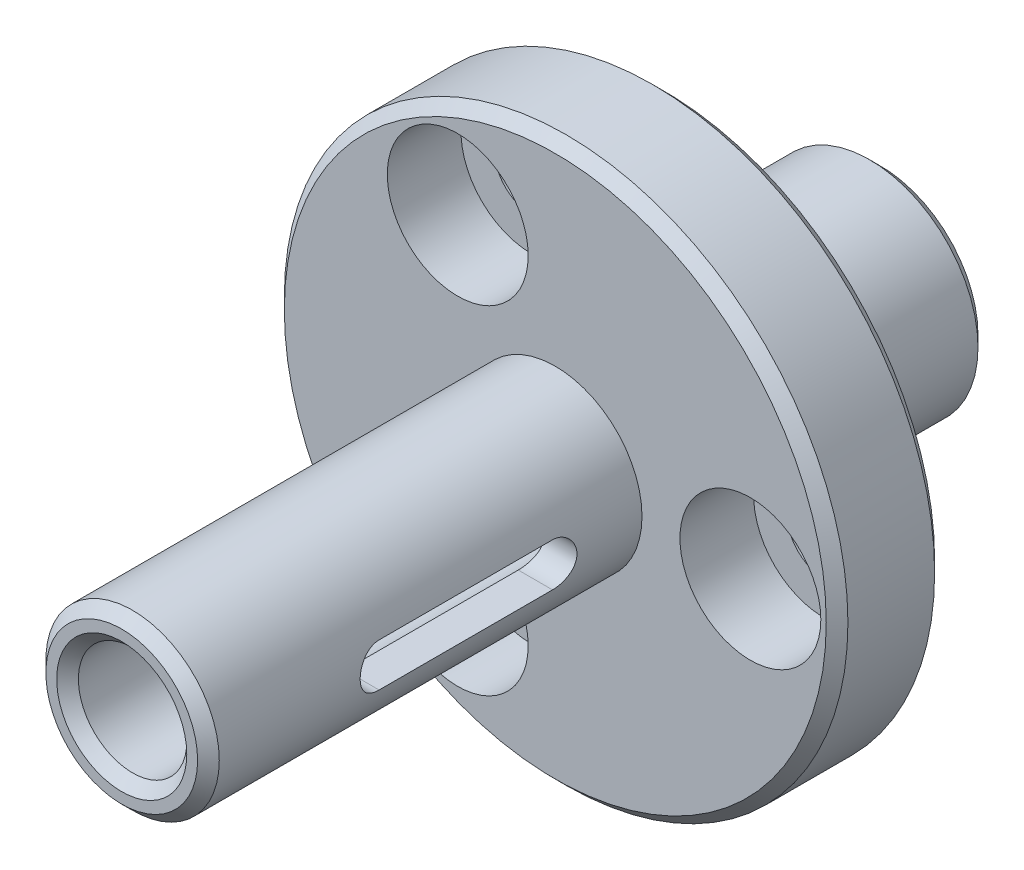
from build123d import *

# Parameters (mm, degrees)
SKETCH1_R                                           = 5
BOSS_EXTRUDE1_DEPTH                                 = 10
SKETCH2_R                                           = 13
BOSS_EXTRUDE2_DEPTH                                 = 5
SKETCH3_R                                           = 4
BOSS_EXTRUDE3_DEPTH                                 = 20
SKETCH4_R                                           = 2.5
CUT_EXTRUDE1_DEPTH                                  = 30
CBORE_FOR_M3_HEX_SOCKET_HEAD_CAP_SCREW1_D           = 3.4
CBORE_FOR_M3_HEX_SOCKET_HEAD_CAP_SCREW1_CBORE_D     = 6.5
CBORE_FOR_M3_HEX_SOCKET_HEAD_CAP_SCREW1_CBORE_DEPTH = 3.4
CIRPATTERN1_COUNT                                   = 3
CUT_EXTRUDE2_DEPTH                                  = 42.024382994
CHAMFER1_SIZE                                       = 0.5


with BuildPart() as part:
    # Sketch1 → Boss-Extrude1 (new body)
    with BuildSketch(Plane.XY):
        Circle(SKETCH1_R)
    extrude(amount=BOSS_EXTRUDE1_DEPTH)

    # Sketch2 → Boss-Extrude2 (add)
    with BuildSketch(Plane.XY.offset(10)):
        Circle(SKETCH2_R)
    extrude(amount=BOSS_EXTRUDE2_DEPTH)

    # Sketch3 → Boss-Extrude3 (add)
    with BuildSketch(Plane.XY.offset(15)):
        Circle(SKETCH3_R)
    extrude(amount=BOSS_EXTRUDE3_DEPTH)

    # Sketch4 → Cut-Extrude1 (cut)
    with BuildSketch(Plane.XY.offset(35)):
        Circle(SKETCH4_R)
    extrude(amount=-CUT_EXTRUDE1_DEPTH, mode=Mode.SUBTRACT)

    # CBORE for M3 Hex Socket Head Cap Screw1 (through all)
    with Locations(Plane.XY.offset(15)):
        with Locations((9, 0)):
            cbore_for_m3_hex_socket_head_cap_screw1 = CounterBoreHole(CBORE_FOR_M3_HEX_SOCKET_HEAD_CAP_SCREW1_D / 2, CBORE_FOR_M3_HEX_SOCKET_HEAD_CAP_SCREW1_CBORE_D / 2, CBORE_FOR_M3_HEX_SOCKET_HEAD_CAP_SCREW1_CBORE_DEPTH)

    # CirPattern1: CBORE for M3 Hex Socket Head Cap Screw1 ×3 about axis
    cirpattern1_axis = Axis((0, 0, 0), (0, 0, 1))
    for i in range(1, CIRPATTERN1_COUNT):
        add(cbore_for_m3_hex_socket_head_cap_screw1.rotate(cirpattern1_axis, i * 360 / CIRPATTERN1_COUNT), mode=Mode.SUBTRACT)

    # Sketch7 → Cut-Extrude2 (cut, through all)
    with BuildSketch(Plane(origin=(4, 0, 0), x_dir=(0, 0, -1), z_dir=(1, 0, 0))):
        with BuildLine():
            Line((-27, 1), (-19, 1))
            ThreePointArc((-19, 1), (-18, 0), (-19, -1))
            Line((-19, -1), (-27, -1))
            ThreePointArc((-27, -1), (-28, 0), (-27, 1))
        make_face()
    extrude(amount=-CUT_EXTRUDE2_DEPTH, mode=Mode.SUBTRACT)

    # Chamfer1
    chamfer1_edges = [part.edges().sort_by_distance(p)[0] for p in [
        (-4, 0, 35),
        (-2.5, 0, 35),
        (-5, 0, 0),
        (-13, 0, 10),
        (-13, 0, 15),
    ]]
    chamfer(chamfer1_edges, length=CHAMFER1_SIZE)


solid = part.part
